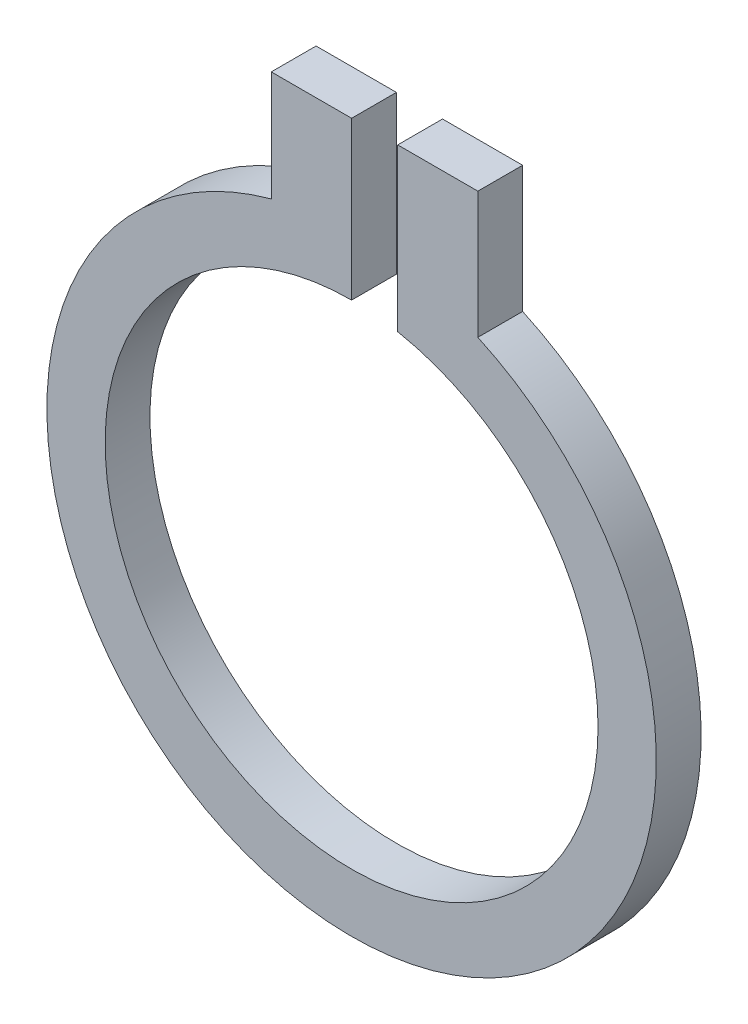
SolidWorks part; units mm, degrees
ref_plane "Front Plane" through (0, 0, 0) normal (0, 0, 1) x (1, 0, 0)
ref_plane "Top Plane" through (0, 0, 0) normal (0, 1, 0) x (1, 0, 0)
ref_plane "Right Plane" through (0, 0, 0) normal (1, 0, 0) x (0, 0, -1)
sketch "Sketch1" plane through (0, 0, 0) normal (0, 0, 1) x (1, 0, 0)
  line L0 (1.0291, 5.4029) -> (1.0291, 9.0149)
  line L1 (1.0291, 9.0149) -> (2.8172, 9.0149)
  line L2 (2.8172, 9.0149) -> (2.8172, 6.189)
  line L3 (0, 5.5) -> (0, 9.0149)
  line L4 (0, 9.0149) -> (-1.7927, 9.0149)
  line L5 (-1.7927, 9.0149) -> (-1.7927, 6.5594)
  arc A0 (-1.7927, 6.5594) -> (2.8172, 6.189) centre (0, 0) ccw
  arc A1 (0, 5.5) -> (1.0291, 5.4029) centre (0, 0) ccw
  dimension "D1" = 11
  dimension "D2" = 13.6
extrude "Boss-Extrude1" add sketch "Sketch1" along normal blind 1
